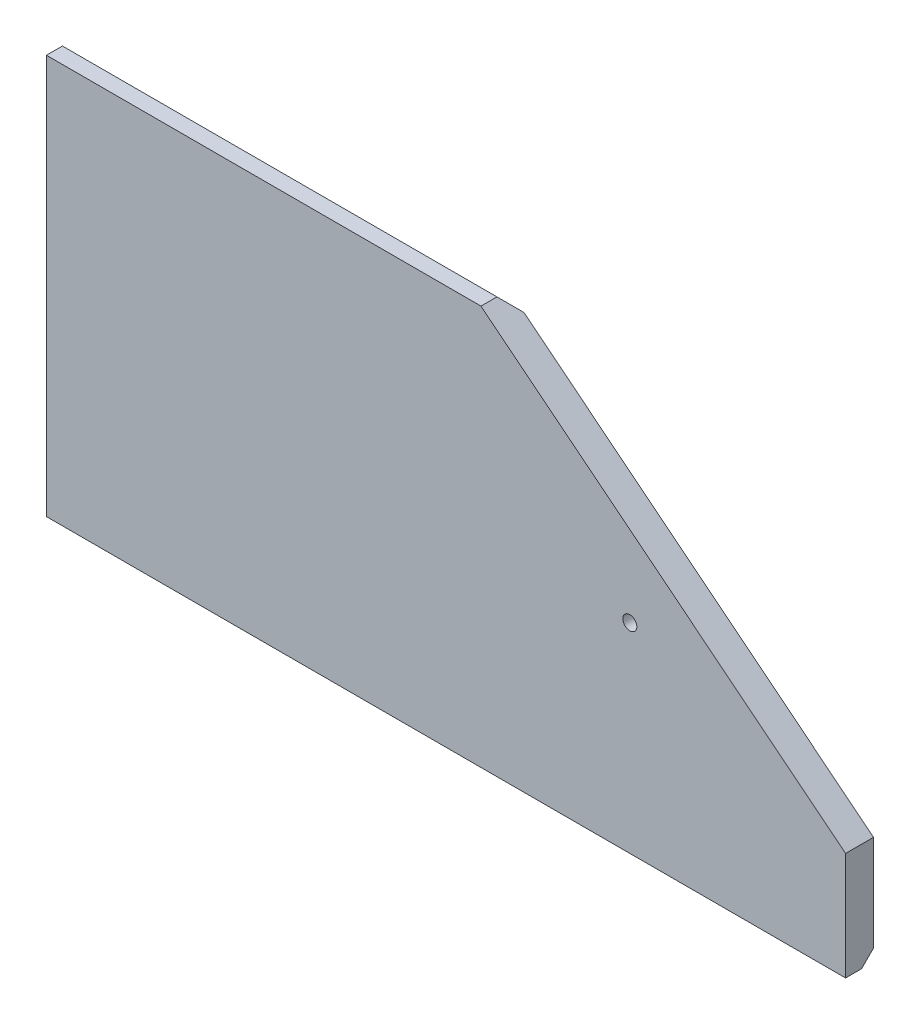
from build123d import *

# Parameters (mm, degrees)
SKETCH1_W           = 1000
SKETCH1_H           = 500
BOSS_EXTRUDE1_DEPTH = 35
M20_TAPPED_HOLE1_D  = 17.5
CHAMFER1_SIZE       = 15
CUT_EXTRUDE3_DEPTH  = 1130.97787589


with BuildPart() as part:
    # Sketch1 → Boss-Extrude1 (new body)
    with BuildSketch(Plane.XY):
        with Locations((-500, -275)):
            Rectangle(SKETCH1_W, SKETCH1_H)
    extrude(amount=-BOSS_EXTRUDE1_DEPTH)

    # M20 Tapped Hole1 (through all)
    with Locations(Plane(origin=(-30, -275, 0), x_dir=(1, 0, 0), z_dir=(0, 0, 1))):
        with Locations((0, 0), (-240, 0)):
            Hole(M20_TAPPED_HOLE1_D / 2)

    # Chamfer1
    chamfer1_edges = [part.edges().sort_by_distance(p)[0] for p in [
        (-500, -525, -35),
        (-500, -25, -35),
    ]]
    chamfer(chamfer1_edges, length=CHAMFER1_SIZE)

    # Sketch9 → Cut-Extrude3 (cut, through all)
    with BuildSketch(Plane.XY):
        Polygon((-500, 10), (0, 10), (0, -390), align=None)
    extrude(amount=-CUT_EXTRUDE3_DEPTH, mode=Mode.SUBTRACT)


solid = part.part
